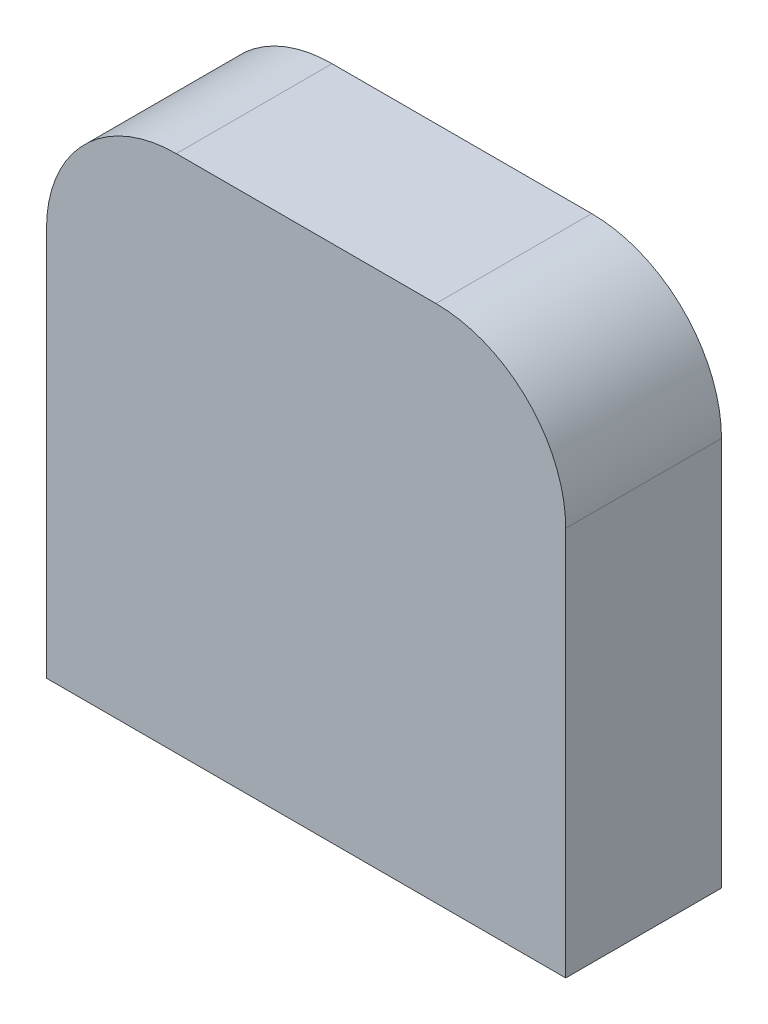
SolidWorks part; units mm, degrees
ref_plane "Front Plane" through (0, 0, 0) normal (0, 0, 1) x (1, 0, 0)
ref_plane "Top Plane" through (0, 0, 0) normal (0, 1, 0) x (1, 0, 0)
ref_plane "Right Plane" through (0, 0, 0) normal (1, 0, 0) x (0, 0, -1)
sketch "Sketch1" plane through (0, 0, 0) normal (0, 0, 1) x (1, 0, 0)
  line L1 (0, 0) -> (40, 0)
  line L2 (0, 0) -> (0, 30)
  line L3 (10, 40) -> (30, 40)
  line L4 (40, 0) -> (40, 30)
  arc A0 (40, 30) -> (30, 40) centre (30, 30) ccw
  arc A1 (0, 30) -> (10, 40) centre (10, 30) cw
  point P9 (0, 40)
  dimension "D3" = 10
  dimension "D1" = 40
  dimension "D2" = 40
extrude "Boss-Extrude1" add sketch "Sketch1" along normal blind 12
